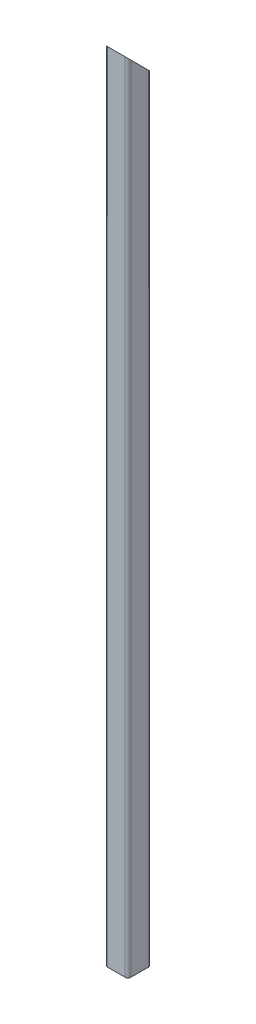
from build123d import *

# Parameters (mm, degrees)
EXTRUDE_1_DEPTH     = 1775
CUT_EXTRUDE_1_DEPTH = 1777.104710103
EXTRUDE_2_DEPTH     = 5
SKETCH_4_W          = 596.189257656
SKETCH_4_H          = 322.935847897
CUT_EXTRUDE_2_DEPTH = 1777.104710103
EXTRUDE_3_DEPTH     = 10


with BuildPart() as part:
    # 草图1 → 凸台-拉伸1 (new body)
    with BuildSketch(Plane(origin=(0, 0, 0), x_dir=(1, 0, 0), z_dir=(0, 1, 0))):
        with BuildLine():
            Line((-19, -12.278106509), (19, -12.278106509))
            ThreePointArc((19, -12.278106509), (23.242640687, -10.520747196), (25, -6.278106509))
            Line((25, -6.278106509), (25, 31.721893491))
            ThreePointArc((25, 31.721893491), (23.242640687, 35.964534178), (19, 37.721893491))
            Line((19, 37.721893491), (-19, 37.721893491))
            ThreePointArc((-19, 37.721893491), (-23.242640687, 35.964534178), (-25, 31.721893491))
            Line((-25, 31.721893491), (-25, -6.278106509))
            ThreePointArc((-25, -6.278106509), (-23.242640687, -10.520747196), (-19, -12.278106509))
        make_face()
        with BuildLine():
            Line((-19, -7.278106509), (19, -7.278106509))
            ThreePointArc((19, -7.278106509), (19.707106781, -6.98521329), (20, -6.278106509))
            Line((20, -6.278106509), (20, 31.721893491))
            ThreePointArc((20, 31.721893491), (19.707106781, 32.429000272), (19, 32.721893491))
            Line((19, 32.721893491), (-19, 32.721893491))
            ThreePointArc((-19, 32.721893491), (-19.707106781, 32.429000272), (-20, 31.721893491))
            Line((-20, 31.721893491), (-20, -6.278106509))
            ThreePointArc((-20, -6.278106509), (-19.707106781, -6.98521329), (-19, -7.278106509))
        make_face(mode=Mode.SUBTRACT)
    extrude(amount=EXTRUDE_1_DEPTH)

    # 草图2 → 切除-拉伸1 (cut, through all)
    with BuildSketch(Plane(origin=(25, 0, 0), x_dir=(0, 0, -1), z_dir=(1, 0, 0))):
        Polygon((-12.278106509, 1775), (37.721893491, 1775), (37.721893491, 1725), align=None)
    extrude(amount=-CUT_EXTRUDE_1_DEPTH, mode=Mode.SUBTRACT)

    # 草图3 → 凸台-拉伸2 (add)
    with BuildSketch(Plane.XZ):
        with BuildLine():
            Line((-25, 6.278106509), (-25, -31.721893491))
            ThreePointArc((-25, -31.721893491), (-23.242640687, -35.964534178), (-19, -37.721893491))
            Line((-19, -37.721893491), (19, -37.721893491))
            ThreePointArc((19, -37.721893491), (23.242640687, -35.964534178), (25, -31.721893491))
            Line((25, -31.721893491), (25, 6.278106509))
            ThreePointArc((25, 6.278106509), (23.242640687, 10.520747196), (19, 12.278106509))
            Line((19, 12.278106509), (-19, 12.278106509))
            ThreePointArc((-19, 12.278106509), (-23.242640687, 10.520747196), (-25, 6.278106509))
        make_face()
    extrude(amount=-EXTRUDE_2_DEPTH)

    # 草图4 → 切除-拉伸2 (cut, through all)
    with BuildSketch(Plane(origin=(25, 0, 0), x_dir=(0, 0, -1), z_dir=(1, 0, 0))):
        with Locations((-43.170849414, -111.467923949)):
            Rectangle(SKETCH_4_W, SKETCH_4_H)
    extrude(amount=-CUT_EXTRUDE_2_DEPTH, mode=Mode.SUBTRACT)

    # 草图5 → 凸台-拉伸3 (add)
    with BuildSketch(Plane.XZ.offset(-50)):
        with BuildLine():
            Line((-25, 6.278106509), (-25, -31.721893491))
            ThreePointArc((-25, -31.721893491), (-23.242640687, -35.964534178), (-19, -37.721893491))
            Line((-19, -37.721893491), (19, -37.721893491))
            ThreePointArc((19, -37.721893491), (23.242640687, -35.964534178), (25, -31.721893491))
            Line((25, -31.721893491), (25, 6.278106509))
            ThreePointArc((25, 6.278106509), (23.242640687, 10.520747196), (19, 12.278106509))
            Line((19, 12.278106509), (-19, 12.278106509))
            ThreePointArc((-19, 12.278106509), (-23.242640687, 10.520747196), (-25, 6.278106509))
        make_face()
    extrude(amount=-EXTRUDE_3_DEPTH)


solid = part.part
